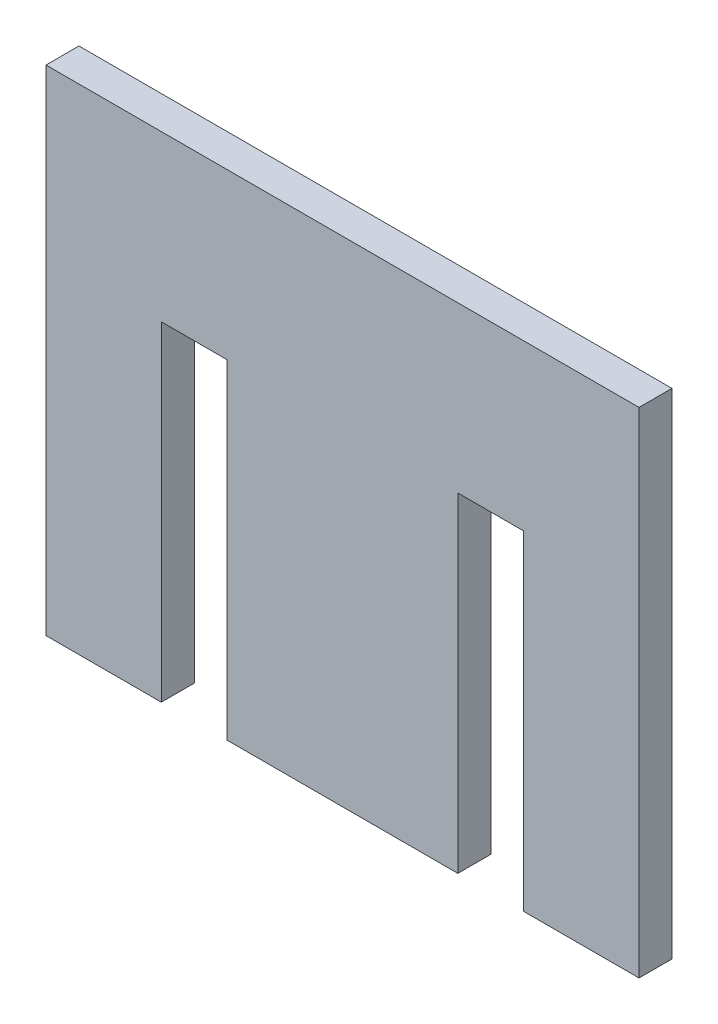
SolidWorks part; units mm, degrees
ref_plane "前视基准面" through (0, 0, 0) normal (0, 0, 1) x (1, 0, 0)
ref_plane "上视基准面" through (0, 0, 0) normal (0, 1, 0) x (1, 0, 0)
ref_plane "右视基准面" through (0, 0, 0) normal (1, 0, 0) x (0, 0, -1)
sketch "草图1" plane through (0, 0, 0) normal (0, 0, 1) x (1, 0, 0)
  line L1 (-90, -75) -> (90, -75)
  line L2 (-90, -75) -> (-90, 75)
  line L3 (-90, 75) -> (90, 75)
  line L4 (90, -75) -> (90, 75)
  line L5 (-90, -75) -> (90, 75) construction
  line L6 (-90, 75) -> (90, -75) construction
  point P0 (0, 0)
  dimension "D1" = 180
  dimension "D2" = 150
extrude "凸台-拉伸1" add sketch "草图1" along normal blind 10
sketch "草图2" plane through (0, 0, 10) normal (0, 0, 1) x (1, 0, 0)
  line L0 (-90, -75) -> (90, -75) construction
  line L1 (-55, -75) -> (-35, -75)
  line L2 (-55, -75) -> (-55, 25)
  line L3 (-55, 25) -> (-35, 25)
  line L4 (-35, -75) -> (-35, 25)
  line L5 (-90, 75) -> (-90, -75) construction
  dimension "D1" = 20
  dimension "D2" = 100
  dimension "D3" = 35
extrude "切除-拉伸1" cut sketch "草图2" against normal up to next
mirror "镜向1" about plane through (0, 0, 0) normal (1, 0, 0) of "切除-拉伸1"
